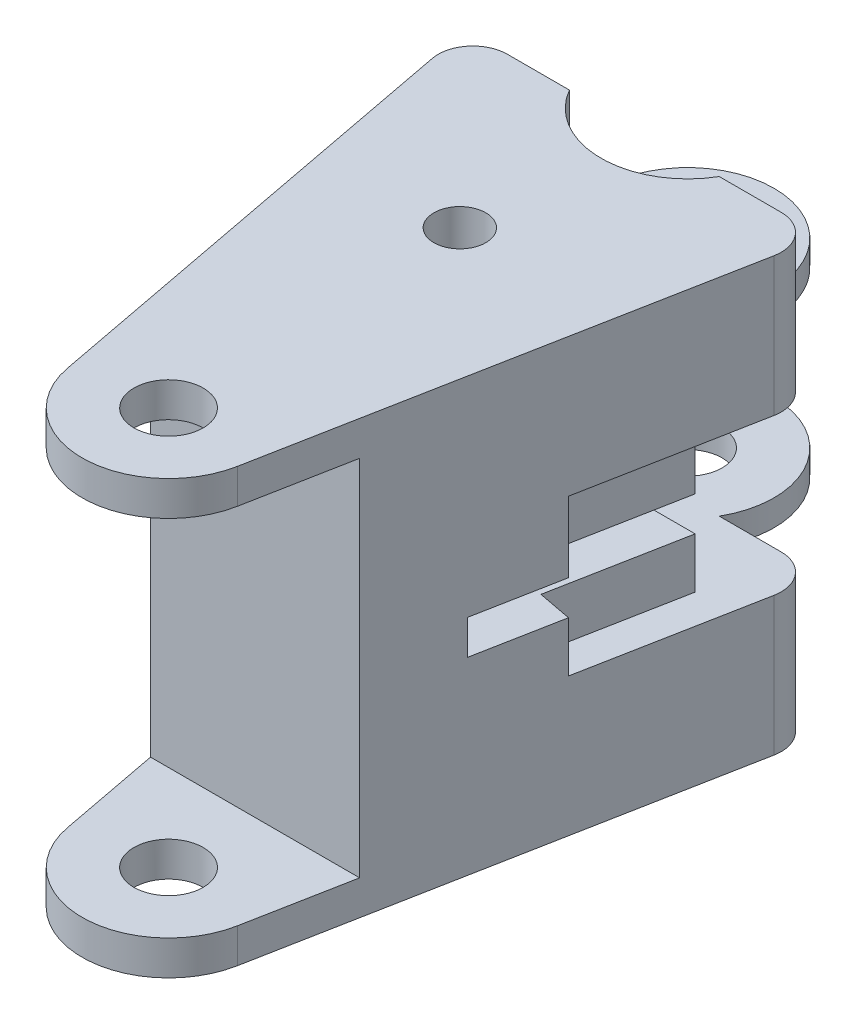
from build123d import *

# Parameters (mm, degrees)
BOSS_EXTRUDE1_DEPTH     = 25
SKETCH2_R               = 2
CUT_EXTRUDE1_DEPTH      = 45.234732103
FILLET1_R               = 2
FILLET2_R               = 2
CUT_EXTRUDE2_START      = -6.5
SKETCH3_R               = 5
CUT_EXTRUDE2_DEPTH      = 6.5
SKETCH4_R               = 5
CUT_EXTRUDE3_DEPTH      = 6.5
CUT_EXTRUDE4_DEPTH      = 45.13919265
CUT_EXTRUDE4_DEPTH_BACK = 45.13919265
SKETCH5_W               = 10
SKETCH5_H               = 21
SKETCH5_W_2             = 12
SKETCH5_H_2             = 9
SKETCH7_W               = 8
SKETCH7_H               = 9
CUT_EXTRUDE5_DEPTH      = 2
CUT_EXTRUDE6_DEPTH      = 189.558524252
CUT_EXTRUDE6_DEPTH_BACK = 189.558524252
SKETCH8_R               = 1.5
CUT_EXTRUDE7_DEPTH      = 46.578505635
CUT_EXTRUDE7_DEPTH_BACK = 46.578505635
SKETCH9_W               = 12.618942776
SKETCH9_H               = 2


with BuildPart() as part:
    # Sketch1 → Boss-Extrude1 (new body)
    with BuildSketch(Plane(origin=(0, 0, 0), x_dir=(1, 0, 0), z_dir=(0, 1, 0))):
        with BuildLine():
            Line((-4.330127019, -2.5), (-10.330127019, -2.5))
            Line((-10.330127019, -2.5), (-4.911624974, -30.935916722))
            ThreePointArc((-4.911624974, -30.935916722), (0, -35), (4.911624974, -30.935916722))
            Line((4.911624974, -30.935916722), (10.330127019, -2.5))
            Line((10.330127019, -2.5), (4.330127019, -2.5))
            ThreePointArc((4.330127019, -2.5), (0, 5), (-4.330127019, -2.5))
        make_face()
    extrude(amount=BOSS_EXTRUDE1_DEPTH)

    # Sketch2 → Cut-Extrude1 (cut, through all)
    with BuildSketch(Plane(origin=(0, 25, 0), x_dir=(1, 0, 0), z_dir=(0, 1, 0))):
        with Locations(Location((0, 0, 0), (0, 0, 270))):
            Circle(SKETCH2_R)
        with Locations(Location((0, -30, 0), (0, 0, 270))):
            Circle(SKETCH2_R)
    extrude(amount=-CUT_EXTRUDE1_DEPTH, mode=Mode.SUBTRACT)

    # Fillet1
    fillet1_edges = [part.edges().sort_by_distance(p)[0] for p in [
        (10.330127019, 12.5, 2.5),
    ]]
    fillet(fillet1_edges, radius=FILLET1_R)

    # Fillet2
    fillet2_edges = [part.edges().sort_by_distance(p)[0] for p in [
        (-10.330127019, 12.5, 2.5),
    ]]
    fillet(fillet2_edges, radius=FILLET2_R)

    # Sketch3 → Cut-Extrude2 (cut)
    with BuildSketch(Plane(origin=(0, 25, 0), x_dir=(1, 0, 0), z_dir=(0, 1, 0)).offset(CUT_EXTRUDE2_START)):
        Circle(SKETCH3_R)
    extrude(amount=CUT_EXTRUDE2_DEPTH, mode=Mode.SUBTRACT)

    # Sketch4 → Cut-Extrude3 (cut)
    with BuildSketch(Plane.XZ):
        Circle(SKETCH4_R)
    extrude(amount=-CUT_EXTRUDE3_DEPTH, mode=Mode.SUBTRACT)

    # Sketch5 → Cut-Extrude4 (cut, two sides: drawn at the far end of the back side and taken through both)
    with BuildSketch(Plane(origin=(0, 0, 0), x_dir=(0, 0, -1), z_dir=(1, 0, 0)).offset(-CUT_EXTRUDE4_DEPTH_BACK)):
        with Locations((-30, 12.5)):
            Rectangle(SKETCH5_W, SKETCH5_H)
        with Locations((-1, 12.5)):
            Rectangle(SKETCH5_W_2, SKETCH5_H_2)
    extrude(amount=CUT_EXTRUDE4_DEPTH + CUT_EXTRUDE4_DEPTH_BACK, mode=Mode.SUBTRACT)

    # Sketch7 → Cut-Extrude5 (cut)
    with BuildSketch(Plane(origin=(10.427871309, 0, 1.987044855), x_dir=(0.18718334440142867, 0, -0.9823249948864665), z_dir=(0.9823249948864665, 0, 0.18718334440142867))):
        with Locations((-9.103153408, 12.5)):
            Rectangle(SKETCH7_W, SKETCH7_H)
    extrude(amount=-CUT_EXTRUDE5_DEPTH, mode=Mode.SUBTRACT)

    # Sketch8 → Cut-Extrude6 (cut, two sides: drawn at the far end of the back side and taken through both)
    with BuildSketch(Plane(origin=(59.598686513, 25, -138.486129663), x_dir=(0.989316462347077, 0, 0.14578387197857126), z_dir=(0, 1, 0)).offset(-CUT_EXTRUDE6_DEPTH_BACK)):
        with Locations(Location((-37.539914968, -158.208081577, 0), (0, 0, 278.382674106))):
            Circle(SKETCH8_R)
    extrude(amount=CUT_EXTRUDE6_DEPTH + CUT_EXTRUDE6_DEPTH_BACK, mode=Mode.SUBTRACT)

    # Sketch9 → Cut-Extrude7 (cut, two sides: drawn at the far end of the back side and taken through both)
    with BuildSketch(Plane(origin=(8.46322132, 0, 1.612678166), x_dir=(0.18718334440142864, 0, -0.9823249948864664), z_dir=(0.9823249948864664, 0, 0.18718334440142864)).offset(-CUT_EXTRUDE7_DEPTH_BACK)):
        with Locations((-11.793727477, 11.917152734)):
            Rectangle(SKETCH9_W, SKETCH9_H)
    extrude(amount=CUT_EXTRUDE7_DEPTH + CUT_EXTRUDE7_DEPTH_BACK, mode=Mode.SUBTRACT)


solid = part.part
